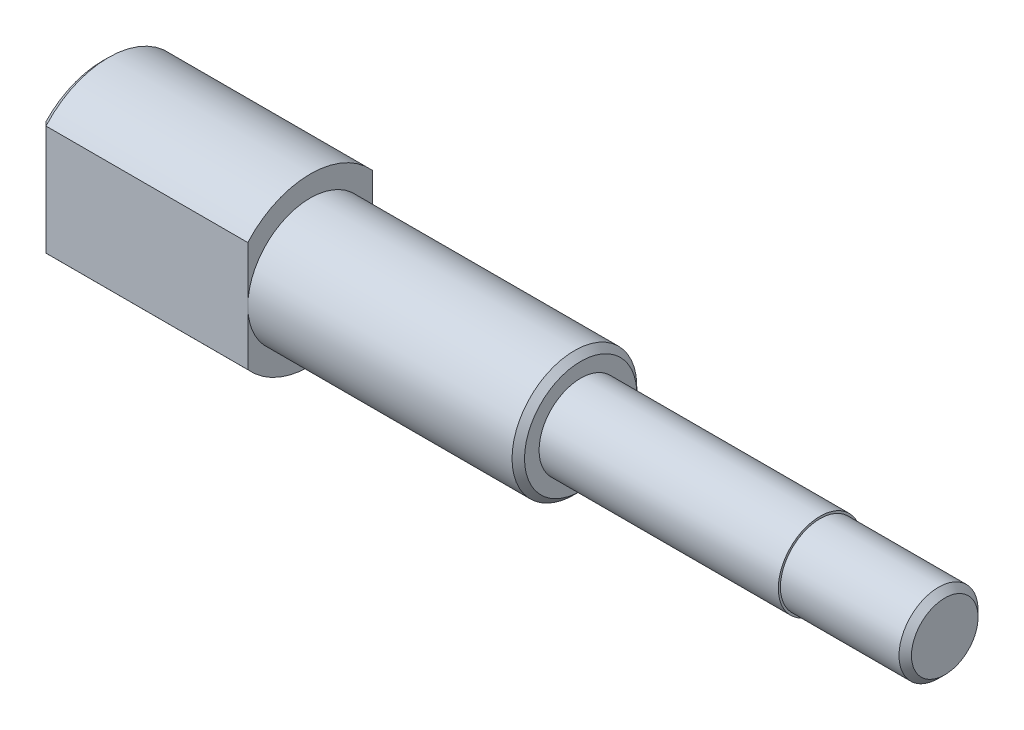
from build123d import *

# Parameters (mm, degrees)
CUT_EXTRUDE1_REACH = 42.893
SKETCH2_W          = 1
SKETCH2_H          = 9.301452206
SKETCH2_H_2        = 8.508093048
CHAMFER2_SIZE      = 0.3


with BuildPart() as part:
    # Sketch1 → Revolve1 (revolve)
    with BuildSketch(Plane.XY, mode=Mode.PRIVATE) as revolve1_sk:
        Polygon((0, 0), (40.5, 0), (40.5, 1.9), (34.5, 1.9), (34.5, 2), (23, 2), (23, 3), (10, 3), (10, 4), (0, 4), align=None)
    revolve(revolve1_sk.sketch.rotate(Axis((0, 0, 0), (1, 0, 0)), 90), axis=Axis((0, 0, 0), (1, 0, 0)))

    # Sketch2 → Cut-Extrude1 (cut, up to next)
    with BuildSketch(Plane.ZY, mode=Mode.PRIVATE) as cut_extrude1_sk1:
        with Locations((-3.5, 0)):
            Rectangle(SKETCH2_W, SKETCH2_H)
    cut_extrude1_tool1 = extrude(cut_extrude1_sk1.sketch, amount=-CUT_EXTRUDE1_REACH, mode=Mode.PRIVATE) & part.part
    # Sketch2 → Cut-Extrude1 (cut, up to next)
    with BuildSketch(Plane.ZY, mode=Mode.PRIVATE) as cut_extrude1_sk2:
        with Locations((3.5, 0)):
            Rectangle(SKETCH2_W, SKETCH2_H_2)
    cut_extrude1_tool2 = extrude(cut_extrude1_sk2.sketch, amount=-CUT_EXTRUDE1_REACH, mode=Mode.PRIVATE) & part.part
    add(cut_extrude1_tool1.solids().sort_by_distance((0, 0, -3.5))[0], mode=Mode.SUBTRACT)
    add(cut_extrude1_tool2.solids().sort_by_distance((0, 0, 3.5))[0], mode=Mode.SUBTRACT)

    # Chamfer2
    chamfer2_edges = [part.edges().sort_by_distance(p)[0] for p in [
        (23, 0, -3),
        (0, 4, 0),
        (0, -4, 0),
        (0, 0, -3),
        (0, 0, 3),
        (40.5, 0, -1.9),
    ]]
    chamfer(chamfer2_edges, length=CHAMFER2_SIZE)


solid = part.part
